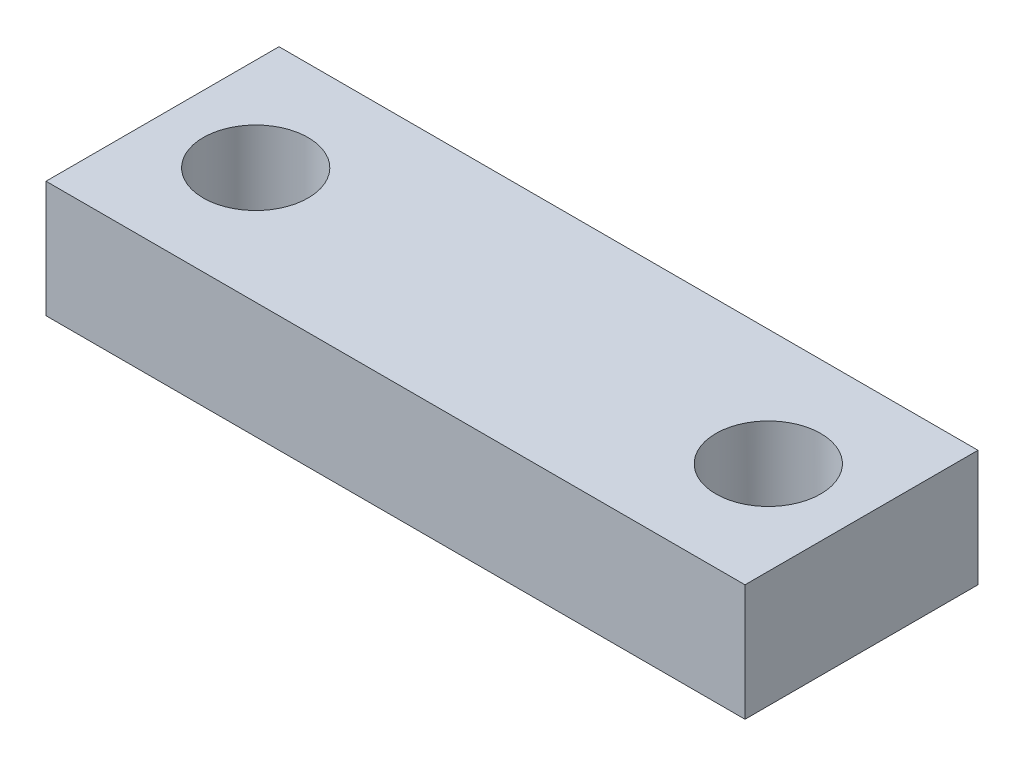
SolidWorks part; units mm, degrees
ref_plane "Front Plane" through (0, 0, 0) normal (0, 0, 1) x (1, 0, 0)
ref_plane "Top Plane" through (0, 0, 0) normal (0, 1, 0) x (1, 0, 0)
ref_plane "Right Plane" through (0, 0, 0) normal (1, 0, 0) x (0, 0, -1)
sketch "Sketch1" plane through (0, 0, 0) normal (0, 1, 0) x (1, 0, 0)
  line L1 (-15, 5) -> (15, 5)
  line L2 (-15, 5) -> (-15, -5)
  line L3 (-15, -5) -> (15, -5)
  line L4 (15, 5) -> (15, -5)
  line L5 (-15, 5) -> (15, -5) construction
  line L6 (-15, -5) -> (15, 5) construction
  point P0 (0, 0)
  dimension "D1" = 30
  dimension "D2" = 10
extrude "Boss-Extrude1" add sketch "Sketch1" along normal blind 5
sketch "Sketch2" plane through (0, 5, 0) normal (0, 1, 0) x (1, 0, 0)
  line L0 (0, 0) -> (0, -50000) construction
  line L1 (0, 0) -> (50000, 0) construction
  circle A0 centre (-11, 0) radius 2.25
  circle A1 centre (11, 0) radius 2.25
  dimension "D1" = 22
  dimension "D2" = 4.5
extrude "Cut-Extrude1" cut sketch "Sketch2" against normal blind 10
